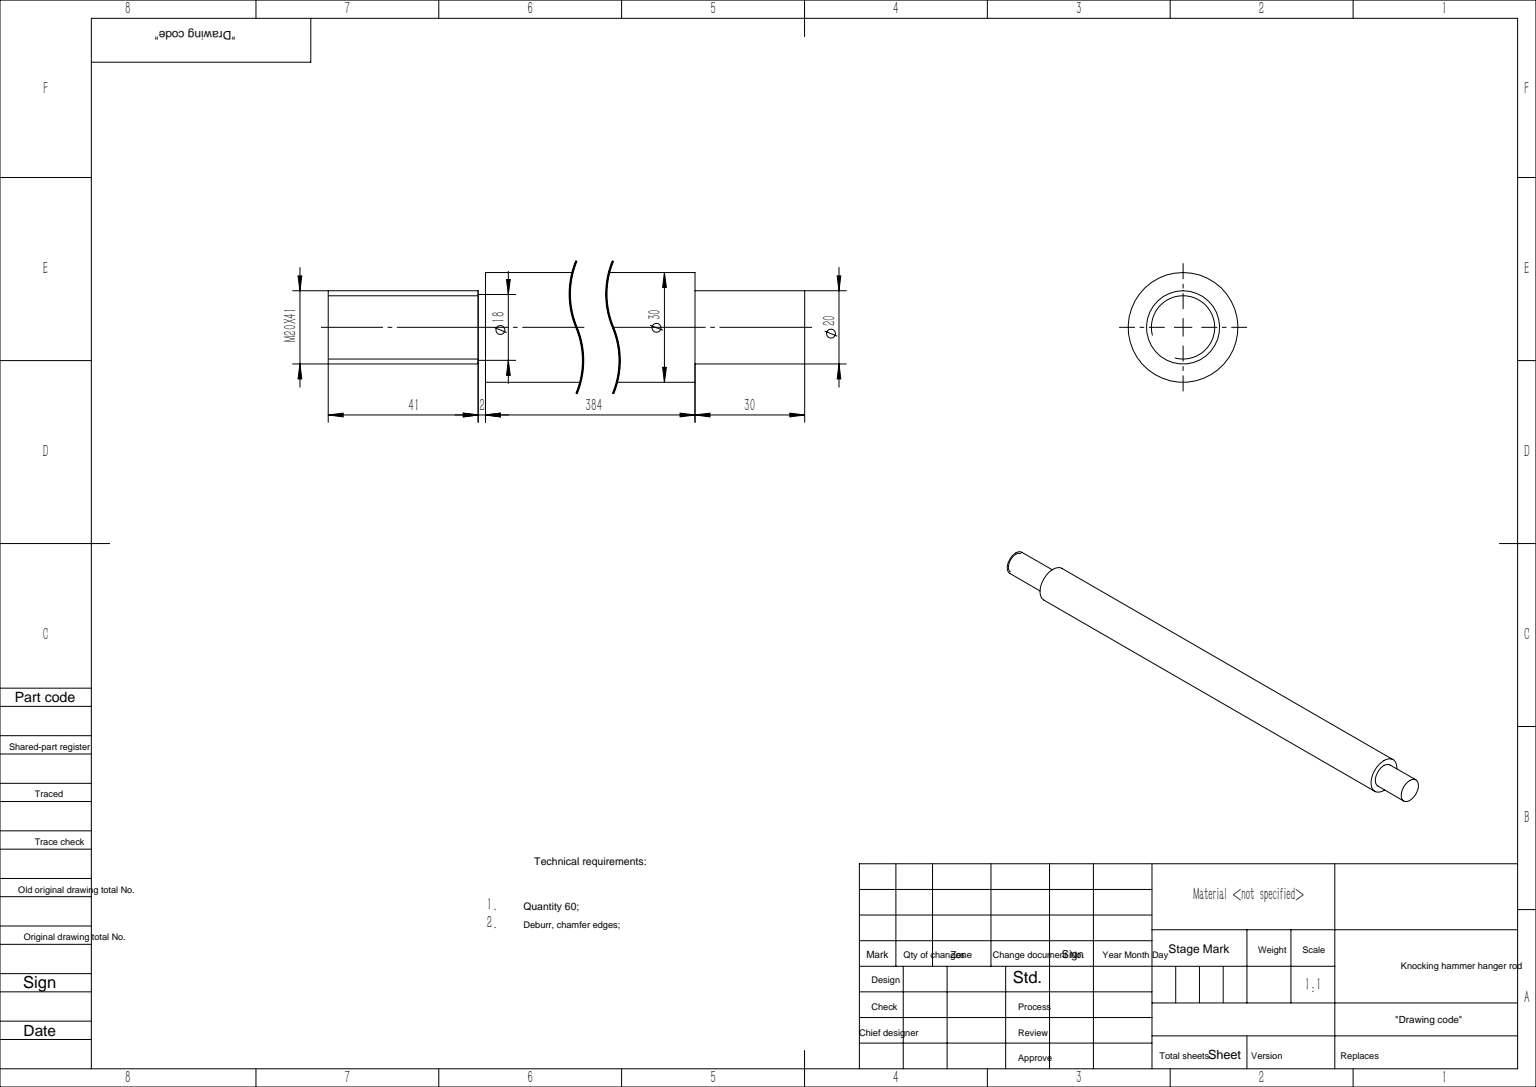
from build123d import *

# Parameters (mm, degrees)
SKETCH_2_R          = 10
SKETCH_2_R_2        = 9
CUT_EXTRUDE_1_DEPTH = 2


with BuildPart() as part:
    # 草图1 → 旋转1 (revolve)
    with BuildSketch(Plane.XY):
        Polygon((0, 0), (0, 10), (43, 10), (43, 15), (427, 15), (427, 10), (457, 10), (457, 0), align=None)
    revolve(axis=Axis((457, 0, 0), (-1, 0, 0)))

    # 草图2 → 切除-拉伸1 (cut)
    with BuildSketch(Plane.ZY.offset(-43)):
        with Locations(Location((0, 0, 0), (0, 0, 90))):
            Circle(SKETCH_2_R)
        with Locations(Location((0, 0, 0), (0, 0, 270))):
            Circle(SKETCH_2_R_2, mode=Mode.SUBTRACT)
    extrude(amount=CUT_EXTRUDE_1_DEPTH, mode=Mode.SUBTRACT)


solid = part.part
